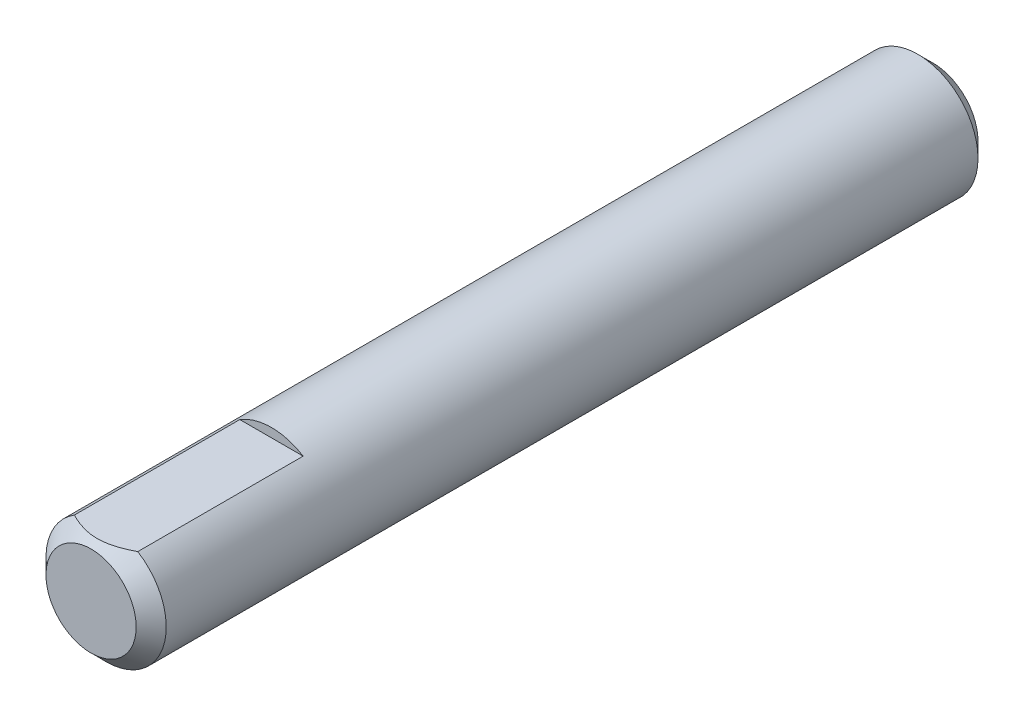
SolidWorks part; units mm, degrees
ref_plane "Front Plane" through (0, 0, 0) normal (0, 0, 1) x (1, 0, 0)
ref_plane "Top Plane" through (0, 0, 0) normal (0, 1, 0) x (1, 0, 0)
ref_plane "Right Plane" through (0, 0, 0) normal (1, 0, 0) x (0, 0, -1)
sketch "Sketch1" plane through (0, 0, 0) normal (0, 0, 1) x (1, 0, 0)
  circle A0 centre (0, 0) radius 2
  dimension "D1" = 4
extrude "Boss-Extrude1" add sketch "Sketch1" along normal blind 28
chamfer "Chamfer1" distance 0.5 angle 45 2 edges at (2, 0, 0) (2, 0, 28)
sketch "Sketch3" plane through (0, 0, 28) normal (0, 0, 1) x (1, 0, 0)
  line L1 (-4.961, 3.9018) -> (5.0189, 3.9018)
  line L2 (-4.961, 3.9018) -> (-4.961, 1.7)
  line L3 (-4.961, 1.7) -> (5.0189, 1.7)
  line L4 (5.0189, 3.9018) -> (5.0189, 1.7)
  dimension "D1" = 1.7
extrude "Cut-Extrude1" cut sketch "Sketch3" against normal blind 6
